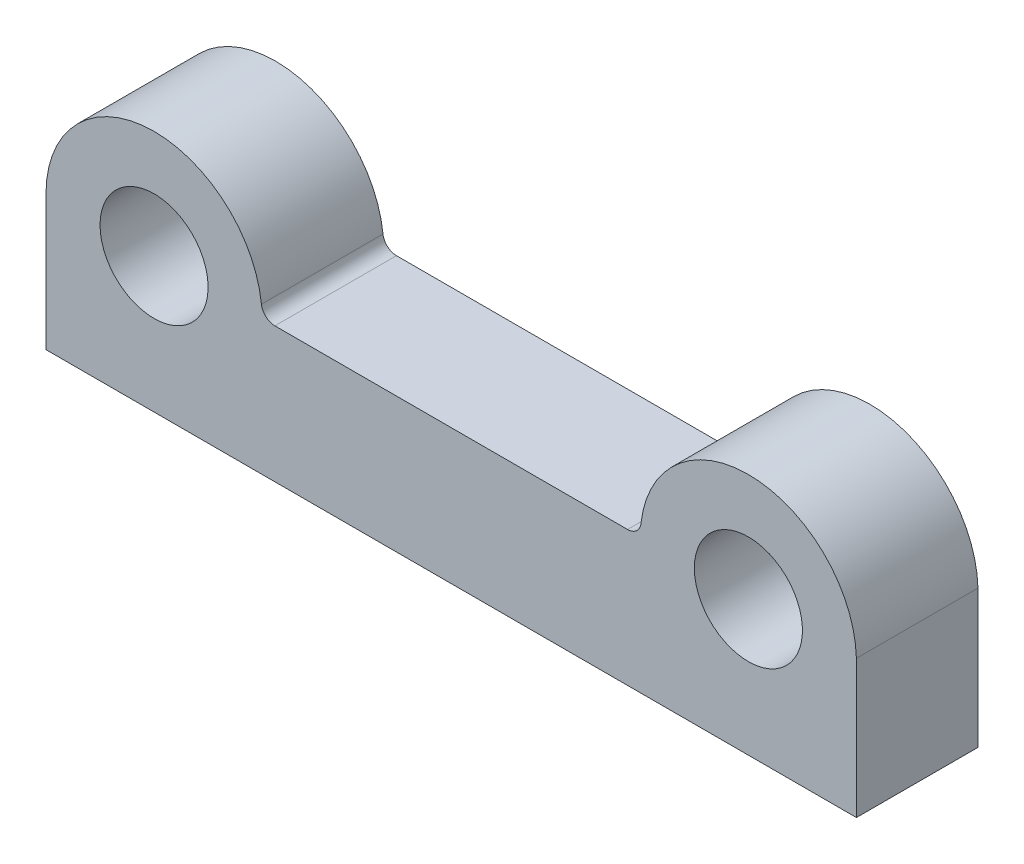
SolidWorks part; units mm, degrees
ref_plane "Front Plane" through (0, 0, 0) normal (0, 0, 1) x (1, 0, 0)
ref_plane "Top Plane" through (0, 0, 0) normal (0, 1, 0) x (1, 0, 0)
ref_plane "Right Plane" through (0, 0, 0) normal (1, 0, 0) x (0, 0, -1)
other "Configuration Table"
sketch "Sketch1" plane through (0, 0, 0) normal (0, 0, 1) x (1, 0, 0)
  line L0 (0, 246.6074) -> (0, -149.8588) construction
  line L1 (-245.7938, 0) -> (266.9117, 0) construction
  line L2 (-300, 0) -> (-300, -100)
  line L3 (-300, -100) -> (300, -100)
  line L4 (300, -100) -> (299.9717, 2.1271)
  line L5 (-130.5573, 0) -> (130.5573, 0)
  circle A0 centre (-220, 0) radius 40
  circle A1 centre (220, 0) radius 40
  arc A2 (-140.4954, 8.8889) -> (-300, 0) centre (-220, 0) ccw
  arc A3 (299.9729, -2.0828) -> (140.4954, 8.8889) centre (220, 0) ccw
  arc A4 (130.5573, 0) -> (140.4954, 8.8889) centre (130.5573, 10) ccw
  arc A5 (-130.5573, 0) -> (-140.4954, 8.8889) centre (-130.5573, 10) cw
  point P18 (140, 0)
  point P21 (-140, 0)
  dimension "D1" = 80
  dimension "D3" = 160
  dimension "D4" = 160
  dimension "D6" = 10
  dimension "D2" = 220
  dimension "D5" = 100
extrude "Boss-Extrude2" add sketch "Sketch1" along normal blind 90 contours L5 A5 A2 L2 L3 L4 A3 A4 A1 A0
